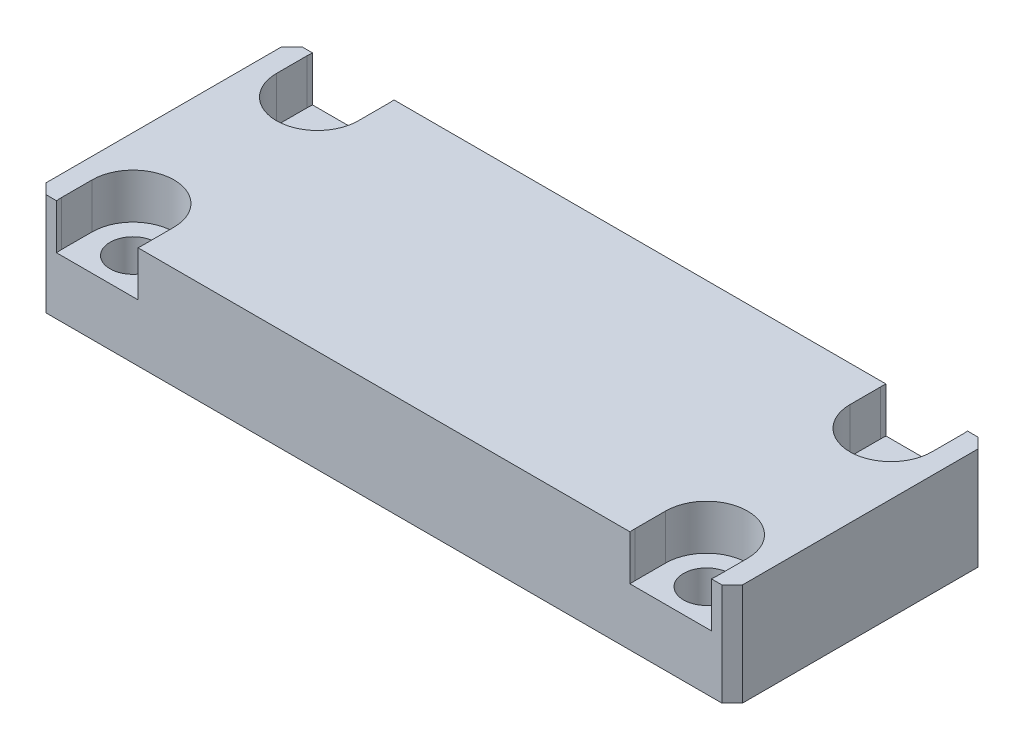
from build123d import *

# Parameters (mm, degrees)
SKETCH_1_W                   = 68
SKETCH_1_H                   = 25
EXTRUDE_1_DEPTH              = 5
HOLE_WIZARD_M4_1_D           = 4.5
HOLE_WIZARD_M4_1_CBORE_D     = 8
HOLE_WIZARD_M4_1_CBORE_DEPTH = 4.4
CUT_EXTRUDE_1_DEPTH          = 4.4
CHAMFER_1_SIZE               = 1


with BuildPart() as part:
    # 草图1 → 凸台-拉伸1 (new, symmetric)
    with BuildSketch(Plane(origin=(0, 0, 0), x_dir=(1, 0, 0), z_dir=(0, 1, 0))):
        Rectangle(SKETCH_1_W, SKETCH_1_H)
    extrude(amount=EXTRUDE_1_DEPTH, both=True)

    # M4 六角凹头螺钉的柱形沉头孔1 (through all)
    with Locations(Plane(origin=(0, 5, 0), x_dir=(1, 0, 0), z_dir=(0, 1, 0))):
        with Locations((-28, 9), (-28, -9), (28, 9), (28, -9)):
            CounterBoreHole(HOLE_WIZARD_M4_1_D / 2, HOLE_WIZARD_M4_1_CBORE_D / 2, HOLE_WIZARD_M4_1_CBORE_DEPTH)

    # 草图4 → 切除-拉伸1 (cut)
    with BuildSketch(Plane(origin=(0, 5, 0), x_dir=(1, 0, 0), z_dir=(0, 1, 0))):
        with BuildLine():
            Line((-32, 9), (-32, 12))
            ThreePointArc((-32, 12), (-28, 16), (-24, 12))
            Line((-24, 12), (-24, 9))
            ThreePointArc((-24, 9), (-28, 5), (-32, 9))
        make_face()
        with BuildLine():
            Line((-32, -9), (-32, -12))
            ThreePointArc((-32, -12), (-28, -16), (-24, -12))
            Line((-24, -12), (-24, -9))
            ThreePointArc((-24, -9), (-28, -5), (-32, -9))
        make_face()
        with BuildLine():
            Line((32, 9), (32, 12))
            ThreePointArc((32, 12), (28, 16), (24, 12))
            Line((24, 12), (24, 9))
            ThreePointArc((24, 9), (28, 5), (32, 9))
        make_face()
        with BuildLine():
            Line((32, -9), (32, -12))
            ThreePointArc((32, -12), (28, -16), (24, -12))
            Line((24, -12), (24, -9))
            ThreePointArc((24, -9), (28, -5), (32, -9))
        make_face()
    extrude(amount=-CUT_EXTRUDE_1_DEPTH, mode=Mode.SUBTRACT)

    # 倒角1
    chamfer_1_edges = [part.edges().sort_by_distance(p)[0] for p in [
        (34, 0, 12.5),
        (-34, 0, 12.5),
        (-34, 0, -12.5),
        (34, 0, -12.5),
    ]]
    chamfer(chamfer_1_edges, length=CHAMFER_1_SIZE)


solid = part.part
